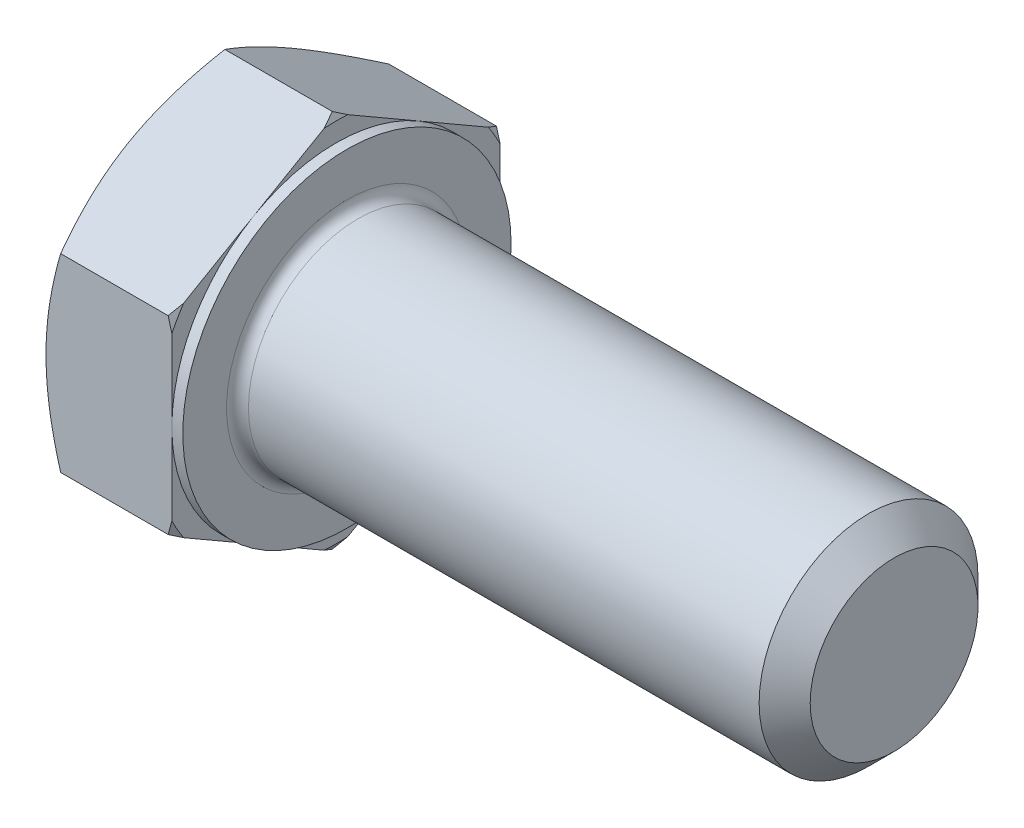
from build123d import *

# Parameters (mm, degrees)
EXTRUDE_360_DEPTH = 7.5
SKETCH_4_W        = 0.6
SKETCH_4_H        = 11.392304845
CHAMFER_1921_SIZE = 1.4
FILLET_1966_R     = 0.6


with BuildPart() as part:
    # 草图1 → Extrude 360 (new body)
    with BuildSketch(Plane(origin=(0, 0, 0), x_dir=(0, 0, -1), z_dir=(1, 0, 0))):
        Polygon((9, 5.196152423), (9, -5.196152423), (0, -10.392304845), (-9, -5.196152423), (-9, 5.196152423), (0, 10.392304845), align=None)
    extrude(amount=EXTRUDE_360_DEPTH)

    # 草图2 → 凸台-旋转1 (revolve)
    with BuildSketch(Plane.XY, mode=Mode.PRIVATE) as revolve_1_sk:
        Polygon((0, 0), (37.5, 0), (37.5, 4.4845), (37.5, 6), (0, 6), align=None)
    revolve(revolve_1_sk.sketch.rotate(Axis((0, 0, 0), (1, 0, 0)), 90), axis=Axis((0, 0, 0), (1, 0, 0)))

    # 草图3 → 切除-旋转1 (revolve, cut)
    with BuildSketch(Plane.XY):
        Polygon((0, 9), (3.690598923, 15.392304845), (3.690598923, 20.392304845), (-10, 20.392304845), (-10, 9), align=None)
    revolve(axis=Axis((0, 0, 0), (1, 0, 0)), mode=Mode.SUBTRACT)

    # 草图5 → 切除-旋转2 (revolve, cut)
    with BuildSketch(Plane.XY):
        Polygon((7.5, 9), (3.809401077, 15.392304845), (3.809401077, 20.392304845), (13.809401077, 20.392304845), (13.809401077, 9), align=None)
    revolve(axis=Axis((0, 0, 0), (1, 0, 0)), mode=Mode.SUBTRACT)

    # 草图4 → 切除-旋转3 (revolve, cut)
    with BuildSketch(Plane.XY, mode=Mode.PRIVATE) as cut_revolve_3_sk:
        with Locations((7.2, 14.696152423)):
            Rectangle(SKETCH_4_W, SKETCH_4_H)
    revolve(cut_revolve_3_sk.sketch.rotate(Axis((0, 0, 0), (1, 0, 0)), 270), axis=Axis((0, 0, 0), (1, 0, 0)), mode=Mode.SUBTRACT)

    # Chamfer 1921
    chamfer_1921_edges = [part.edges().sort_by_distance(p)[0] for p in [
        (37.5, 0, -6),
    ]]
    chamfer(chamfer_1921_edges, length=CHAMFER_1921_SIZE)

    # Fillet 1966
    fillet_1966_edges = [part.edges().sort_by_distance(p)[0] for p in [
        (7.5, 0, -6),
    ]]
    fillet(fillet_1966_edges, radius=FILLET_1966_R)


solid = part.part
